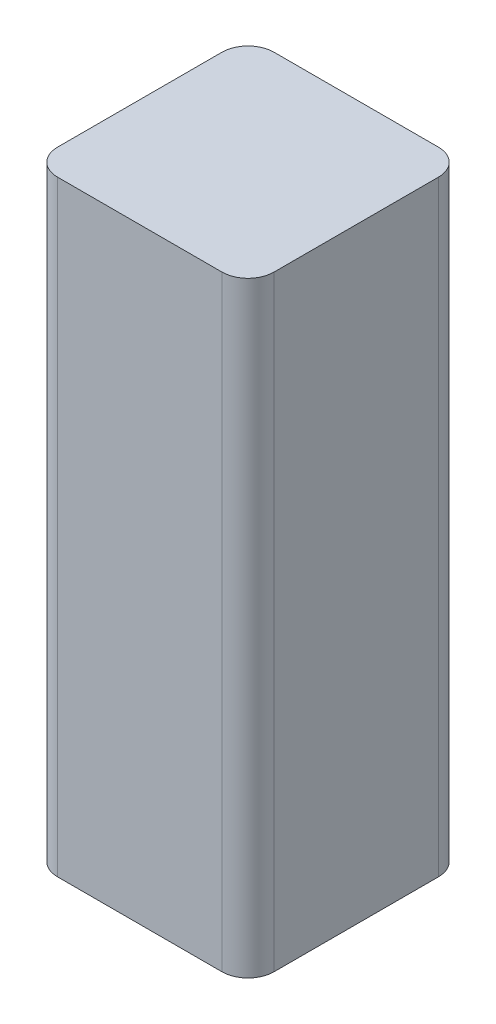
SolidWorks part; units mm, degrees
ref_plane "Front" through (0, 0, 0) normal (0, 0, 1) x (1, 0, 0)
ref_plane "Top" through (0, 0, 0) normal (0, 1, 0) x (1, 0, 0)
ref_plane "Right" through (0, 0, 0) normal (1, 0, 0) x (0, 0, -1)
sketch "草图1" plane through (0, 0, 0) normal (0, 1, 0) x (1, 0, 0)
  line L0 (-19, -7.2781) -> (19, -7.2781)
  line L1 (-19, -12.2781) -> (19, -12.2781)
  line L2 (-25, -6.2781) -> (-25, 31.7219)
  line L3 (-19, 37.7219) -> (19, 37.7219)
  line L4 (25, -6.2781) -> (25, 31.7219)
  line L5 (20, -6.2781) -> (20, 31.7219)
  line L6 (-19, 32.7219) -> (19, 32.7219)
  line L11 (-20, -6.2781) -> (-20, 31.7219)
  arc A0 (-19, -12.2781) -> (-25, -6.2781) centre (-19, -6.2781) cw
  arc A1 (19, -12.2781) -> (25, -6.2781) centre (19, -6.2781) ccw
  arc A2 (19, 37.7219) -> (25, 31.7219) centre (19, 31.7219) cw
  arc A3 (-25, 31.7219) -> (-19, 37.7219) centre (-19, 31.7219) cw
  arc A4 (19, -7.2781) -> (20, -6.2781) centre (19, -6.2781) ccw
  arc A5 (19, 32.7219) -> (20, 31.7219) centre (19, 31.7219) cw
  arc A6 (-20, 31.7219) -> (-19, 32.7219) centre (-19, 31.7219) cw
  arc A7 (-19, -7.2781) -> (-20, -6.2781) centre (-19, -6.2781) cw
  point P9 (25, -12.2781)
  point P12 (25, 37.7219)
  point P15 (-25, 37.7219)
  dimension "D3" = 6
  dimension "D1" = 50
  dimension "D2" = 50
  dimension "D4" = 5
extrude "凸台-拉伸1" add sketch "草图1" along normal blind 140
sketch "草图2" plane through (0, 140, 0) normal (0, 1, 0) x (1, 0, 0)
  line L4 (-19, -12.2781) -> (19, -12.2781)
  line L5 (25, -6.2781) -> (25, 31.7219)
  line L6 (19, 37.7219) -> (-19, 37.7219)
  line L7 (-25, 31.7219) -> (-25, -6.2781)
  line L8 (-19, -12.2781) -> (19, -12.2781)
  line L9 (25, -6.2781) -> (25, 31.7219)
  line L10 (19, 37.7219) -> (-19, 37.7219)
  line L11 (-25, 31.7219) -> (-25, -6.2781)
  arc A4 (-25, -6.2781) -> (-19, -12.2781) centre (-19, -6.2781) ccw
  arc A5 (19, -12.2781) -> (25, -6.2781) centre (19, -6.2781) ccw
  arc A6 (25, 31.7219) -> (19, 37.7219) centre (19, 31.7219) ccw
  arc A7 (-19, 37.7219) -> (-25, 31.7219) centre (-19, 31.7219) ccw
  arc A8 (-25, -6.2781) -> (-19, -12.2781) centre (-19, -6.2781) ccw
  arc A9 (19, -12.2781) -> (25, -6.2781) centre (19, -6.2781) ccw
  arc A10 (25, 31.7219) -> (19, 37.7219) centre (19, 31.7219) ccw
  arc A11 (-19, 37.7219) -> (-25, 31.7219) centre (-19, 31.7219) ccw
  dimension "D1" = 0
extrude "凸台-拉伸2" add sketch "草图2" against normal blind 5
